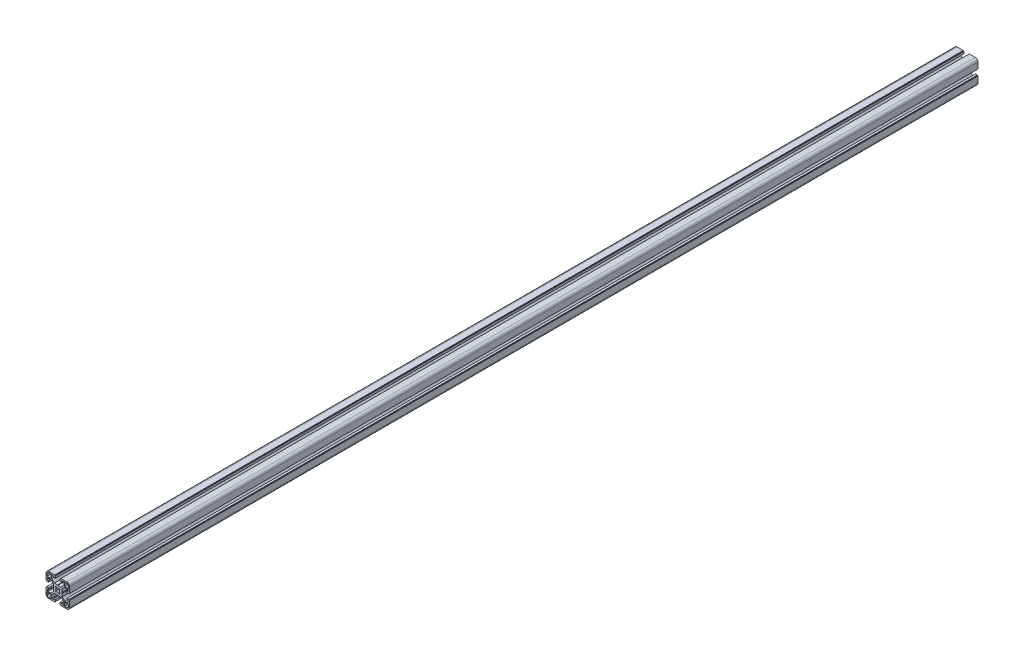
SolidWorks part; units mm, degrees
material "6061 GB/T6892-2006"
ref_plane "前视" through (0, 0, 0) normal (0, 0, 1) x (1, 0, 0)
ref_plane "上视" through (0, 0, 0) normal (0, 1, 0) x (1, 0, 0)
ref_plane "右视" through (0, 0, 0) normal (1, 0, 0) x (0, 0, -1)
sketch "草图1" plane through (0, 0, 0) normal (0, 0, 1) x (1, 0, 0)
  line L0 (-18.9995, -4.1003) -> (-18.9995, -5.1003)
  line L1 (-18.9995, -5.1003) -> (-19.9995, -5.1003)
  line L2 (-19.9995, -5.1003) -> (-19.9995, -15.5003)
  line L3 (-15.4995, -20.0003) -> (-5.0995, -20.0003)
  line L4 (-5.0995, -20.0003) -> (-5.0995, -19.0003)
  line L5 (-5.0995, -19.0003) -> (-4.0995, -19.0003)
  line L6 (-4.0995, -19.0003) -> (-4.0995, -15.5003)
  line L7 (-4.0995, -15.5003) -> (-6.5995, -15.5003)
  line L8 (-6.5995, -15.5003) -> (-6.5995, -16.5003)
  line L9 (-7.5995, -17.5003) -> (-9.7995, -17.5003)
  line L10 (-10.2995, -17.0003) -> (-10.2995, -11.9973)
  line L11 (-10.2995, -11.9973) -> (-5.9025, -7.6003)
  line L12 (-5.9025, -7.6003) -> (-0.5195, -7.6003)
  line L13 (-0.5195, -7.6003) -> (0.0005, -7.3003)
  line L14 (0.0005, -7.3003) -> (0.5195, -7.6003)
  line L15 (0.5195, -7.6003) -> (5.9035, -7.6003)
  line L16 (5.9035, -7.6003) -> (10.3005, -11.9973)
  line L17 (10.3005, -11.9973) -> (10.3005, -17.0003)
  line L18 (9.8005, -17.5003) -> (7.6005, -17.5003)
  line L19 (6.6005, -16.5003) -> (6.6005, -15.5003)
  line L20 (6.6005, -15.5003) -> (4.1005, -15.5003)
  line L21 (4.1005, -15.5003) -> (4.1005, -19.0003)
  line L22 (4.1005, -19.0003) -> (5.1005, -19.0003)
  line L23 (5.1005, -19.0003) -> (5.1005, -20.0003)
  line L24 (5.1005, -20.0003) -> (15.5005, -20.0003)
  line L25 (20.0005, -15.5003) -> (20.0005, -5.1003)
  line L26 (20.0005, -5.1003) -> (19.0005, -5.1003)
  line L27 (19.0005, -5.1003) -> (19.0005, -4.1003)
  line L28 (19.0005, -4.1003) -> (15.5005, -4.1003)
  line L29 (15.5005, -4.1003) -> (15.5005, -6.6003)
  line L30 (15.5005, -6.6003) -> (16.5005, -6.6003)
  line L31 (17.5005, -7.6003) -> (17.5005, -9.8003)
  line L32 (17.0005, -10.3003) -> (11.9975, -10.3003)
  line L33 (11.9975, -10.3003) -> (7.6005, -5.9033)
  line L34 (7.6005, -5.9033) -> (7.6005, -0.5203)
  line L35 (7.6005, -0.5203) -> (7.3005, -0.0003)
  line L36 (7.3005, -0.0003) -> (7.6005, 0.5197)
  line L37 (7.6005, 0.5197) -> (7.6005, 5.9027)
  line L38 (7.6005, 5.9027) -> (11.9975, 10.2997)
  line L39 (11.9975, 10.2997) -> (17.0005, 10.2997)
  line L40 (17.5005, 9.7997) -> (17.5005, 7.5997)
  line L41 (16.5005, 6.5997) -> (15.5005, 6.5997)
  line L42 (15.5005, 6.5997) -> (15.5005, 4.0997)
  line L43 (15.5005, 4.0997) -> (19.0005, 4.0997)
  line L44 (19.0005, 4.0997) -> (19.0005, 5.0997)
  line L45 (19.0005, 5.0997) -> (20.0005, 5.0997)
  line L46 (20.0005, 5.0997) -> (20.0005, 15.4997)
  line L47 (15.5005, 19.9997) -> (5.1005, 19.9997)
  line L48 (5.1005, 19.9997) -> (5.1005, 18.9997)
  line L49 (5.1005, 18.9997) -> (4.1005, 18.9997)
  line L50 (4.1005, 18.9997) -> (4.1005, 15.4997)
  line L51 (4.1005, 15.4997) -> (6.6005, 15.4997)
  line L52 (7.6005, 17.4997) -> (9.8005, 17.4997)
  line L53 (10.3005, 16.9997) -> (10.3005, 11.9967)
  line L54 (10.3005, 11.9967) -> (5.9035, 7.5997)
  line L55 (5.9035, 7.5997) -> (0.5195, 7.5997)
  line L56 (0.5195, 7.5997) -> (0.0005, 7.2997)
  line L57 (0.0005, 7.2997) -> (-0.5195, 7.5997)
  line L58 (-0.5195, 7.5997) -> (-5.9025, 7.5997)
  line L59 (-5.9025, 7.5997) -> (-10.2995, 11.9967)
  line L60 (-10.2995, 11.9967) -> (-10.2995, 16.9997)
  line L61 (-9.7995, 17.4997) -> (-7.5995, 17.4997)
  line L62 (-6.5995, 16.4997) -> (-6.5995, 15.4997)
  line L63 (-6.5995, 15.4997) -> (-4.0995, 15.4997)
  line L64 (-4.0995, 15.4997) -> (-4.0995, 18.9997)
  line L65 (-4.0995, 18.9997) -> (-5.0995, 18.9997)
  line L66 (-5.0995, 18.9997) -> (-5.0995, 19.9997)
  line L67 (-5.0995, 19.9997) -> (-15.4995, 19.9997)
  line L68 (-19.9995, 15.4997) -> (-19.9995, 5.0997)
  line L69 (-19.9995, 5.0997) -> (-18.9995, 5.0997)
  line L70 (-18.9995, 5.0997) -> (-18.9995, 4.0997)
  line L71 (-18.9995, 4.0997) -> (-15.4995, 4.0997)
  line L72 (-15.4995, 4.0997) -> (-15.4995, 6.5997)
  line L73 (-15.4995, 6.5997) -> (-16.4995, 6.5997)
  line L74 (-17.4995, 7.5997) -> (-17.4995, 9.7997)
  line L75 (-16.9995, 10.2997) -> (-11.9965, 10.2997)
  line L76 (-11.9965, 10.2997) -> (-7.5995, 5.9027)
  line L77 (-7.5995, 5.9027) -> (-7.5995, 0.5197)
  line L78 (-7.5995, 0.5197) -> (-7.2995, -0.0003)
  line L79 (-7.2995, -0.0003) -> (-7.5995, -0.5203)
  line L80 (-7.5995, -0.5203) -> (-7.5995, -5.9033)
  line L81 (-7.5995, -5.9033) -> (-11.9965, -10.3003)
  line L82 (-11.9965, -10.3003) -> (-16.9995, -10.3003)
  line L83 (-17.4995, -9.8003) -> (-17.4995, -7.6003)
  line L84 (-16.4995, -6.6003) -> (-15.4995, -6.6003)
  line L85 (-15.4995, -6.6003) -> (-15.4995, -4.1003)
  line L86 (-15.4995, -4.1003) -> (-18.9995, -4.1003)
  line L87 (15.5005, -18.0003) -> (11.8005, -18.0003)
  line L88 (11.8005, -18.0003) -> (11.8005, -11.8003)
  line L89 (11.8005, -11.8003) -> (18.0005, -11.8003)
  line L90 (18.0005, -11.8003) -> (18.0005, -15.5003)
  line L91 (18.0005, 11.7997) -> (11.8005, 11.7997)
  line L92 (11.8005, 11.7997) -> (11.8005, 17.9997)
  line L93 (11.8005, 17.9997) -> (15.5005, 17.9997)
  line L94 (18.0005, 15.4997) -> (18.0005, 11.7997)
  line L95 (-1.8145, -2.8753) -> (-3.0044, -4.0665)
  line L96 (-3.0044, -4.0665) -> (-4.0656, -3.0052)
  line L97 (-4.0656, -3.0052) -> (-2.8745, -1.8153)
  line L98 (-2.8745, 1.8147) -> (-4.0644, 3.0058)
  line L99 (-4.0644, 3.0058) -> (-3.0044, 4.0658)
  line L100 (-3.0044, 4.0658) -> (-1.8145, 2.8747)
  line L101 (1.8145, 2.8747) -> (3.0055, 4.0657)
  line L102 (3.0055, 4.0657) -> (4.0666, 3.0045)
  line L103 (4.0666, 3.0045) -> (2.8755, 1.8147)
  line L104 (2.8755, -1.8153) -> (4.0666, -3.0052)
  line L105 (4.0666, -3.0052) -> (3.0055, -4.0663)
  line L106 (3.0055, -4.0663) -> (1.8145, -2.8753)
  line L107 (-17.9995, -15.5003) -> (-17.9995, -11.8003)
  line L108 (-17.9995, -11.8003) -> (-11.7995, -11.8003)
  line L109 (-11.7995, -11.8003) -> (-11.7995, -18.0003)
  line L110 (-11.7995, -18.0003) -> (-15.4995, -18.0003)
  line L111 (-11.7995, 17.9997) -> (-11.7995, 11.7997)
  line L112 (-11.7995, 11.7997) -> (-17.9995, 11.7997)
  line L113 (-17.9995, 11.7997) -> (-17.9995, 15.4997)
  line L114 (-15.4995, 17.9997) -> (-11.7995, 17.9997)
  arc A0 (-19.9995, -15.5003) -> (-15.4995, -20.0003) centre (-15.4995, -15.5003) ccw
  arc A1 (-6.5995, -16.5003) -> (-7.5995, -17.5003) centre (-7.5995, -16.5003) cw
  arc A2 (-9.7995, -17.5003) -> (-10.2995, -17.0003) centre (-9.7995, -17.0003) cw
  arc A3 (10.3005, -17.0003) -> (9.8005, -17.5003) centre (9.8005, -17.0003) cw
  arc A4 (7.6005, -17.5003) -> (6.6005, -16.5003) centre (7.6005, -16.5003) cw
  arc A5 (15.5005, -20.0003) -> (20.0005, -15.5003) centre (15.5005, -15.5003) ccw
  arc A6 (16.5005, -6.6003) -> (17.5005, -7.6003) centre (16.5005, -7.6003) cw
  arc A7 (17.5005, -9.8003) -> (17.0005, -10.3003) centre (17.0005, -9.8003) cw
  arc A8 (17.0005, 10.2997) -> (17.5005, 9.7997) centre (17.0005, 9.7997) cw
  arc A9 (17.5005, 7.5997) -> (16.5005, 6.5997) centre (16.5005, 7.5997) cw
  arc A10 (20.0005, 15.4997) -> (15.5005, 19.9997) centre (15.5005, 15.4997) ccw
  arc A11 (6.6005, 15.4997) -> (6.6005, 16.4997) centre (7.1003, 15.9997) cw
  arc A12 (6.6005, 16.4997) -> (7.6005, 17.4997) centre (7.6005, 16.4997) cw
  arc A13 (9.8005, 17.4997) -> (10.3005, 16.9997) centre (9.8005, 16.9997) cw
  arc A14 (-10.2995, 16.9997) -> (-9.7995, 17.4997) centre (-9.7995, 16.9997) cw
  arc A15 (-7.5995, 17.4997) -> (-6.5995, 16.4997) centre (-7.5995, 16.4997) cw
  arc A16 (-15.4995, 19.9997) -> (-19.9995, 15.4997) centre (-15.4995, 15.4997) ccw
  arc A17 (-16.4995, 6.5997) -> (-17.4995, 7.5997) centre (-16.4995, 7.5997) cw
  arc A18 (-17.4995, 9.7997) -> (-16.9995, 10.2997) centre (-16.9995, 9.7997) cw
  arc A19 (-16.9995, -10.3003) -> (-17.4995, -9.8003) centre (-16.9995, -9.8003) cw
  arc A20 (-17.4995, -7.6003) -> (-16.4995, -6.6003) centre (-16.4995, -7.6003) cw
  arc A21 (18.0005, -15.5003) -> (15.5005, -18.0003) centre (15.5005, -15.5003) cw
  arc A22 (15.5005, 17.9997) -> (18.0005, 15.4997) centre (15.5005, 15.4997) cw
  arc A23 (-2.8745, -1.8153) -> (-2.8745, 1.8147) centre (0.0005, -0.0003) cw
  arc A24 (-1.8145, 2.8747) -> (1.8145, 2.8747) centre (0, -0.0007) cw
  arc A25 (2.8755, 1.8147) -> (2.8755, -1.8153) centre (0.0005, -0.0003) cw
  arc A26 (1.8145, -2.8753) -> (-1.8145, -2.8753) centre (0, 0) cw
  arc A27 (-15.4995, -18.0003) -> (-17.9995, -15.5003) centre (-15.4995, -15.5003) cw
  arc A28 (-17.9995, 15.4997) -> (-15.4995, 17.9997) centre (-15.4995, 15.4997) cw
extrude "凸台-拉伸1" add sketch "草图1" against normal blind 1548
